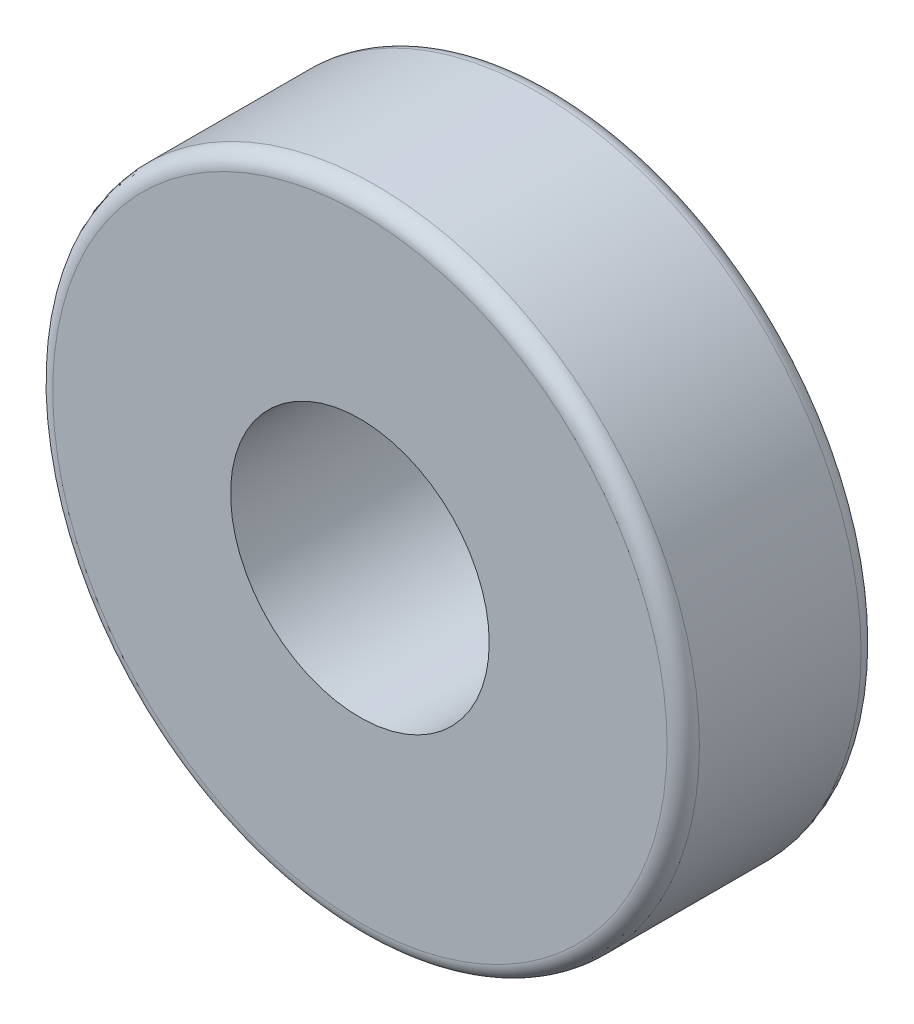
from build123d import *

# Parameters (mm, degrees)
SKETCH_1_R      = 10
SKETCH_1_R_2    = 4
EXTRUDE_1_DEPTH = 6
FILLET_1_R      = 0.5


with BuildPart() as part:
    # 草图1 → 凸台-拉伸1 (new body)
    with BuildSketch(Plane.XY):
        Circle(SKETCH_1_R)
        Circle(SKETCH_1_R_2, mode=Mode.SUBTRACT)
    extrude(amount=EXTRUDE_1_DEPTH)

    # 圆角1
    fillet_1_edges = [part.edges().sort_by_distance(p)[0] for p in [
        (-10, 0, 0),
        (-10, 0, 6),
    ]]
    fillet(fillet_1_edges, radius=FILLET_1_R)


solid = part.part
